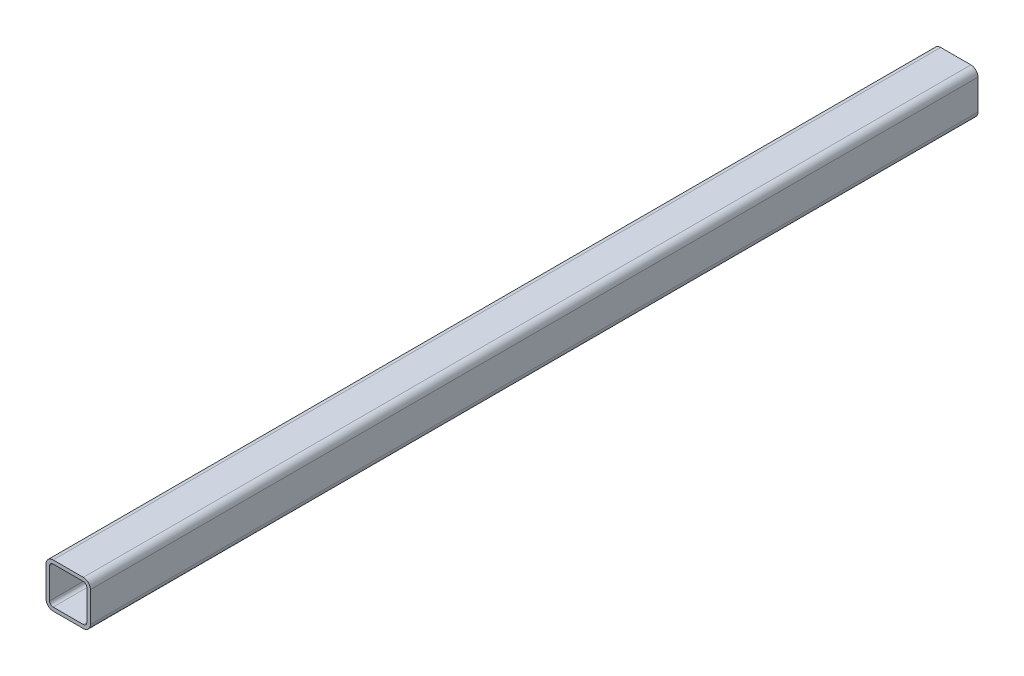
SolidWorks part; units mm, degrees
ref_plane "Front Plane" through (0, 0, 0) normal (0, 0, 1) x (1, 0, 0)
ref_plane "Top Plane" through (0, 0, 0) normal (0, 1, 0) x (1, 0, 0)
ref_plane "Right Plane" through (0, 0, 0) normal (1, 0, 0) x (0, 0, -1)
sketch "Sketch1" plane through (0, 0, 0) normal (0, 0, 1) x (1, 0, 0)
  line L0 (23, 4) -> (23, 21)
  line L1 (4, 0) -> (21, 0)
  line L2 (0, 4) -> (0, 21)
  line L3 (4, 25) -> (21, 25)
  line L4 (25, 4) -> (25, 21)
  line L5 (4, 2) -> (21, 2)
  line L6 (2, 4) -> (2, 21)
  line L7 (4, 23) -> (21, 23)
  arc A0 (4, 0) -> (0, 4) centre (4, 4) cw
  arc A1 (21, 0) -> (25, 4) centre (21, 4) ccw
  arc A2 (21, 25) -> (25, 21) centre (21, 21) cw
  arc A3 (0, 21) -> (4, 25) centre (4, 21) cw
  arc A4 (21, 23) -> (23, 21) centre (21, 21) cw
  arc A5 (21, 2) -> (23, 4) centre (21, 4) ccw
  arc A6 (4, 2) -> (2, 4) centre (4, 4) cw
  arc A7 (2, 21) -> (4, 23) centre (4, 21) cw
  point P7 (0, 0)
  point P10 (25, 0)
  point P15 (0, 25)
  dimension "D3" = 4
  dimension "D1" = 25
  dimension "D2" = 25
  dimension "D4" = 2
extrude "Boss-Extrude1" add sketch "Sketch1" along normal blind 500
